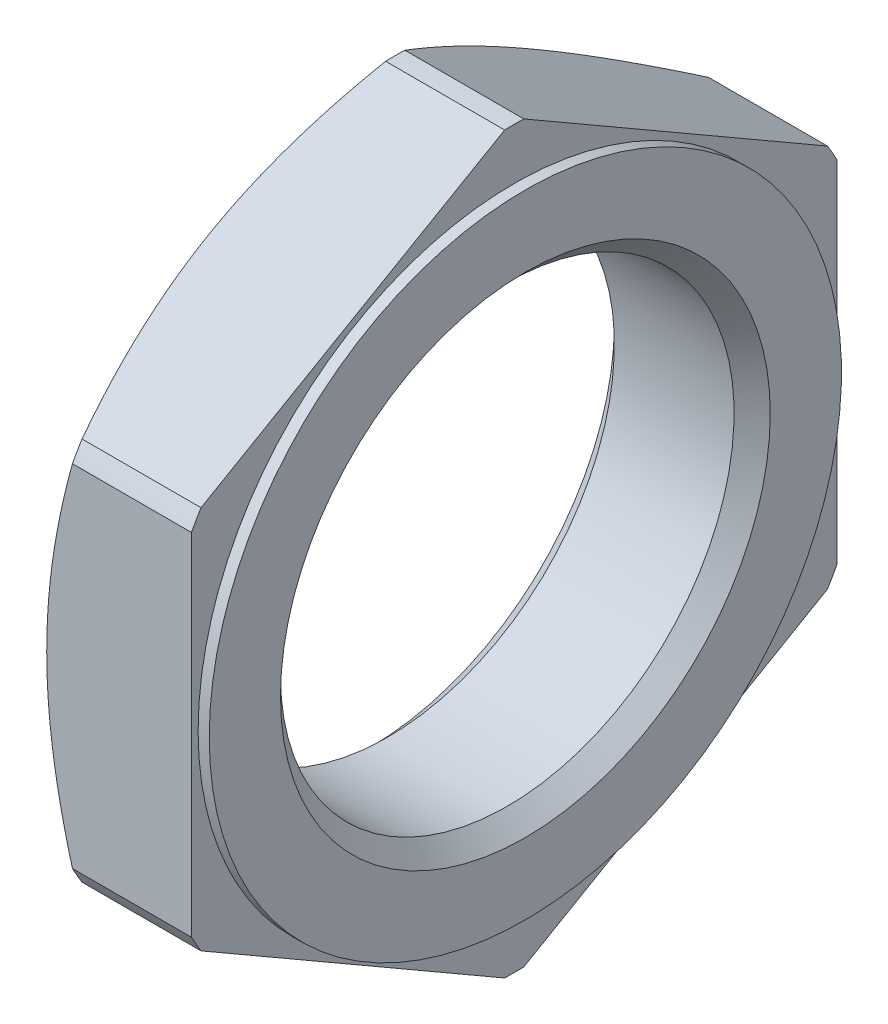
from build123d import *

# Parameters (mm, degrees)
SKETCH_3_W          = 58
SKETCH_3_H          = 58
CUT_EXTRUDE_1_DEPTH = 7
SCALE_1_SCALE       = 0.5


with BuildPart() as part:
    # 草图1 → 旋转1 (revolve)
    with BuildSketch(Plane.XY, mode=Mode.PRIVATE) as revolve_1_sk:
        Polygon((0, 0), (0, 14.5), (1.154700538, 16.5), (6.5, 16.5), (6.5, 14.2), (7, 14.2), (7, 0), align=None)
    revolve(revolve_1_sk.sketch.rotate(Axis((7, 0, 0), (-1, 0, 0)), 270), axis=Axis((7, 0, 0), (-1, 0, 0)))

    # 草图2 → 切除-旋转1 (revolve, cut)
    with BuildSketch(Plane.XY, mode=Mode.PRIVATE) as cut_revolve_1_sk:
        Polygon((0, 0), (0, 11), (0.812, 10.188), (6.188, 10.188), (7, 11), (7, 0), align=None)
    revolve(cut_revolve_1_sk.sketch.rotate(Axis((7, 0, 0), (-1, 0, 0)), 270), axis=Axis((7, 0, 0), (-1, 0, 0)), mode=Mode.SUBTRACT)

    # 草图3 → 切除-拉伸1 (cut)
    with BuildSketch(Plane(origin=(0, 0, 0), x_dir=(0, 0, -1), z_dir=(1, 0, 0))):
        Rectangle(SKETCH_3_W, SKETCH_3_H)
        Polygon((-14.5, -8.371578903), (0, -16.743157806), (14.5, -8.371578903), (14.5, 8.371578903), (0, 16.743157806), (-14.5, 8.371578903), align=None, mode=Mode.SUBTRACT)
    extrude(amount=CUT_EXTRUDE_1_DEPTH, mode=Mode.SUBTRACT)


with BuildPart() as part_1:
    # 缩放比例1: scaled about (3.473718043, 0, 0)
    add(part.part.scale(SCALE_1_SCALE).moved(Location((1.736859021, 0, 0))))


solid = part_1.part
